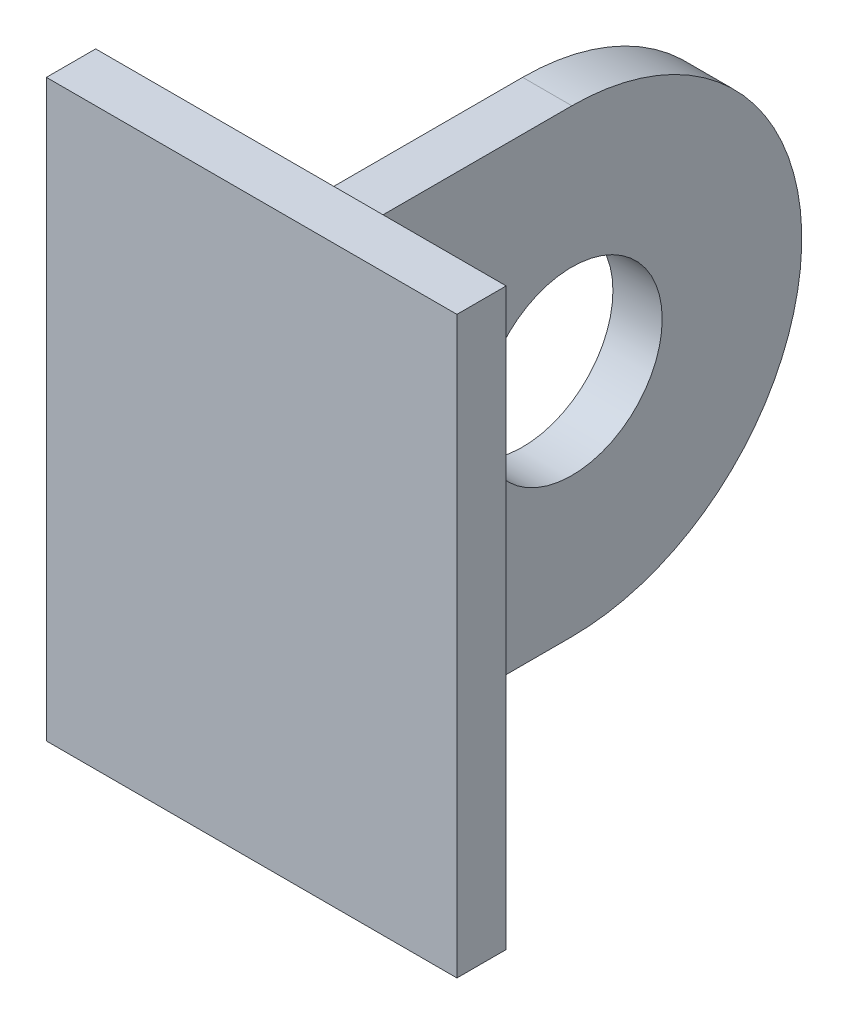
SolidWorks part; units mm, degrees
ref_plane "前视基准面" through (0, 0, 0) normal (0, 0, 1) x (1, 0, 0)
ref_plane "上视基准面" through (0, 0, 0) normal (0, 1, 0) x (1, 0, 0)
ref_plane "右视基准面" through (0, 0, 0) normal (1, 0, 0) x (0, 0, -1)
sketch "草图1" plane through (0, 0, 0) normal (0, 0, 1) x (1, 0, 0)
  line L1 (-12.5, 17.5) -> (12.5, 17.5)
  line L2 (-12.5, 17.5) -> (-12.5, -17.5)
  line L3 (-12.5, -17.5) -> (12.5, -17.5)
  line L4 (12.5, 17.5) -> (12.5, -17.5)
  line L5 (-12.5, 17.5) -> (12.5, -17.5) construction
  line L6 (-12.5, -17.5) -> (12.5, 17.5) construction
  point P0 (0, 0)
  dimension "D1" = 35
  dimension "D2" = 25
extrude "凸台-拉伸1" add sketch "草图1" along normal blind 3
sketch "草图2" plane through (0, 0, 0) normal (1, 0, 0) x (0, 0, -1)
  line L0 (0, 14) -> (15, 14)
  line L1 (0, -17.5) -> (0, 17.5) construction
  line L2 (0, -14) -> (15, -14)
  line L3 (0, 14) -> (0, -14)
  arc A0 (15, 14) -> (15, -14) centre (15, 0) cw
  circle A1 centre (15, 0) radius 5.5
  dimension "D4" = 11
  dimension "D1" = 15
  dimension "D2" = 14
  dimension "D3" = 14
extrude "凸台-拉伸2" add sketch "草图2" along normal mid plane 3 separate body
